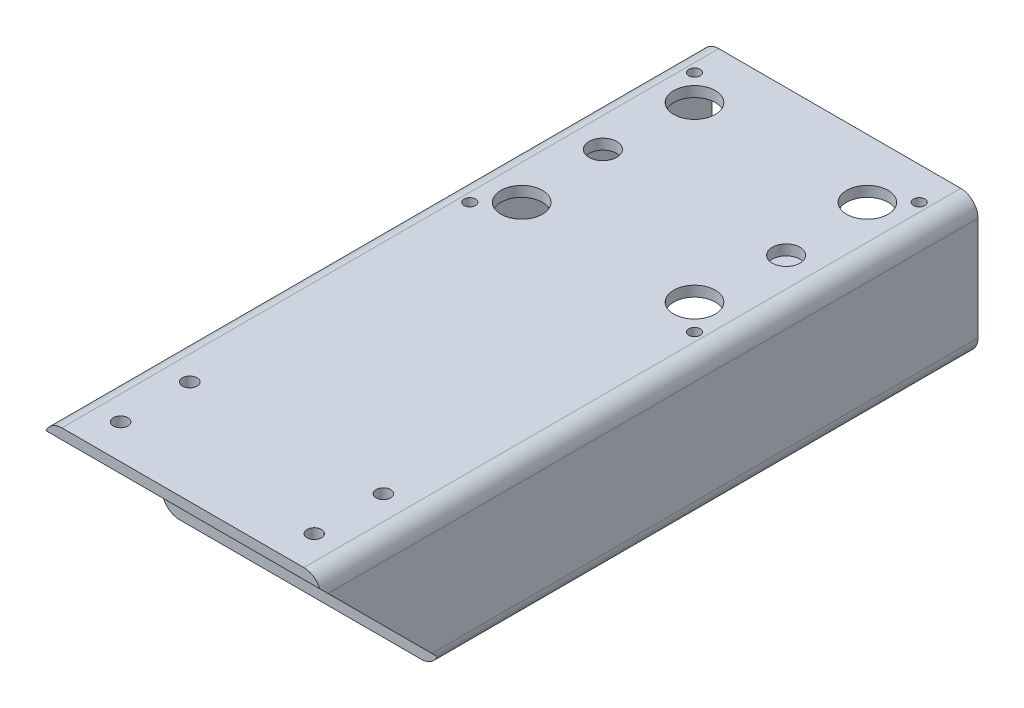
from build123d import *

# Parameters (mm, degrees)
EXTRUDE_1_DEPTH              = 190
SKETCH_6_R                   = 23.25
CUT_EXTRUDE_1_DEPTH          = 3
HOLE_WIZARD_6_5_6_5_1_D      = 6.5
HOLE_WIZARD_12_0_12_1_REACH  = 200.242
HOLE_WIZARD_12_0_12_1_BORE_R = 6
HOLE_WIZARD_M4_1_REACH       = 200.242
HOLE_WIZARD_M4_1_BORE_R      = 1.65
CUT_EXTRUDE_2_DEPTH          = 208.123151772
SKETCH_12_R                  = 5
EXTRUDE_2_DEPTH              = 3
HOLE_WIZARD_M5_1_D           = 4.2
HOLE_WIZARD_M3_1_D           = 2.5
HOLE_WIZARD_M3_1_DEPTH       = 3
CUT_EXTRUDE_3_REACH          = 200.242
SKETCH_17_R                  = 4


with BuildPart() as part:
    # 草图1 → 凸台-拉伸1 (new body)
    with BuildSketch(Plane.XY):
        with BuildLine():
            Line((-35, 20), (35, 20))
            ThreePointArc((35, 20), (38.535533906, 18.535533906), (40, 15))
            Line((40, 15), (40, -15))
            ThreePointArc((40, -15), (38.535533906, -18.535533906), (35, -20))
            Line((35, -20), (-35, -20))
            ThreePointArc((-35, -20), (-38.535533906, -18.535533906), (-40, -15))
            Line((-40, -15), (-40, 15))
            ThreePointArc((-40, 15), (-38.535533906, 18.535533906), (-35, 20))
        make_face()
        with BuildLine():
            Line((-37, 15), (-37, -15))
            ThreePointArc((-37, -15), (-36.414213562, -16.414213562), (-35, -17))
            Line((-35, -17), (35, -17))
            ThreePointArc((35, -17), (36.414213562, -16.414213562), (37, -15))
            Line((37, -15), (37, 15))
            ThreePointArc((37, 15), (36.414213562, 16.414213562), (35, 17))
            Line((35, 17), (-35, 17))
            ThreePointArc((-35, 17), (-36.414213562, 16.414213562), (-37, 15))
        make_face(mode=Mode.SUBTRACT)
    extrude(amount=EXTRUDE_1_DEPTH)

    # 草图6 → 切除-拉伸1 (cut)
    with BuildSketch(Plane.XZ.offset(20)):
        with Locations(Location((0, 42, 0), (0, 0, 270))):
            Circle(SKETCH_6_R)
    extrude(amount=-CUT_EXTRUDE_1_DEPTH, mode=Mode.SUBTRACT)

    # Ø6.5 (6.5) 直径孔1 (through all)
    with Locations(Plane(origin=(0, 20, 0), x_dir=(1, 0, 0), z_dir=(0, 1, 0))):
        with Locations((-25, -17), (25, -17), (25, -67), (-25, -67)):
            Hole(HOLE_WIZARD_6_5_6_5_1_D / 2)

    # Ø12.0 (12) 直径孔1 bore → Ø12.0 (12) 直径孔1 (cut, up to next)
    with BuildSketch(Plane(origin=(0, 20, 0), x_dir=(1, 0, 0), z_dir=(0, 1, 0)), mode=Mode.PRIVATE) as hole_wizard_12_0_12_1_sk1:
        with Locations((-25, -17)):
            Circle(HOLE_WIZARD_12_0_12_1_BORE_R)
    hole_wizard_12_0_12_1_tool1 = extrude(hole_wizard_12_0_12_1_sk1.sketch, amount=-HOLE_WIZARD_12_0_12_1_REACH, mode=Mode.PRIVATE) & part.part
    # Ø12.0 (12) 直径孔1 bore → Ø12.0 (12) 直径孔1 (cut, up to next)
    with BuildSketch(Plane(origin=(0, 20, 0), x_dir=(1, 0, 0), z_dir=(0, 1, 0)), mode=Mode.PRIVATE) as hole_wizard_12_0_12_1_sk2:
        with Locations((25, -17)):
            Circle(HOLE_WIZARD_12_0_12_1_BORE_R)
    hole_wizard_12_0_12_1_tool2 = extrude(hole_wizard_12_0_12_1_sk2.sketch, amount=-HOLE_WIZARD_12_0_12_1_REACH, mode=Mode.PRIVATE) & part.part
    # Ø12.0 (12) 直径孔1 bore → Ø12.0 (12) 直径孔1 (cut, up to next)
    with BuildSketch(Plane(origin=(0, 20, 0), x_dir=(1, 0, 0), z_dir=(0, 1, 0)), mode=Mode.PRIVATE) as hole_wizard_12_0_12_1_sk3:
        with Locations((25, -67)):
            Circle(HOLE_WIZARD_12_0_12_1_BORE_R)
    hole_wizard_12_0_12_1_tool3 = extrude(hole_wizard_12_0_12_1_sk3.sketch, amount=-HOLE_WIZARD_12_0_12_1_REACH, mode=Mode.PRIVATE) & part.part
    # Ø12.0 (12) 直径孔1 bore → Ø12.0 (12) 直径孔1 (cut, up to next)
    with BuildSketch(Plane(origin=(0, 20, 0), x_dir=(1, 0, 0), z_dir=(0, 1, 0)), mode=Mode.PRIVATE) as hole_wizard_12_0_12_1_sk4:
        with Locations((-25, -67)):
            Circle(HOLE_WIZARD_12_0_12_1_BORE_R)
    hole_wizard_12_0_12_1_tool4 = extrude(hole_wizard_12_0_12_1_sk4.sketch, amount=-HOLE_WIZARD_12_0_12_1_REACH, mode=Mode.PRIVATE) & part.part
    add(hole_wizard_12_0_12_1_tool1.solids().sort_by_distance((-25, 20, 17))[0], mode=Mode.SUBTRACT)
    add(hole_wizard_12_0_12_1_tool2.solids().sort_by_distance((25, 20, 17))[0], mode=Mode.SUBTRACT)
    add(hole_wizard_12_0_12_1_tool3.solids().sort_by_distance((25, 20, 67))[0], mode=Mode.SUBTRACT)
    add(hole_wizard_12_0_12_1_tool4.solids().sort_by_distance((-25, 20, 67))[0], mode=Mode.SUBTRACT)

    # M4 螺纹孔1 bore → M4 螺纹孔1 (cut, up to next)
    with BuildSketch(Plane(origin=(0, 20, 0), x_dir=(1, 0, 0), z_dir=(0, 1, 0)), mode=Mode.PRIVATE) as hole_wizard_m4_1_sk1:
        with Locations((-32.5, -9.5)):
            Circle(HOLE_WIZARD_M4_1_BORE_R)
    hole_wizard_m4_1_tool1 = extrude(hole_wizard_m4_1_sk1.sketch, amount=-HOLE_WIZARD_M4_1_REACH, mode=Mode.PRIVATE) & part.part
    # M4 螺纹孔1 bore → M4 螺纹孔1 (cut, up to next)
    with BuildSketch(Plane(origin=(0, 20, 0), x_dir=(1, 0, 0), z_dir=(0, 1, 0)), mode=Mode.PRIVATE) as hole_wizard_m4_1_sk2:
        with Locations((32.5, -9.5)):
            Circle(HOLE_WIZARD_M4_1_BORE_R)
    hole_wizard_m4_1_tool2 = extrude(hole_wizard_m4_1_sk2.sketch, amount=-HOLE_WIZARD_M4_1_REACH, mode=Mode.PRIVATE) & part.part
    # M4 螺纹孔1 bore → M4 螺纹孔1 (cut, up to next)
    with BuildSketch(Plane(origin=(0, 20, 0), x_dir=(1, 0, 0), z_dir=(0, 1, 0)), mode=Mode.PRIVATE) as hole_wizard_m4_1_sk3:
        with Locations((32.5, -74.5)):
            Circle(HOLE_WIZARD_M4_1_BORE_R)
    hole_wizard_m4_1_tool3 = extrude(hole_wizard_m4_1_sk3.sketch, amount=-HOLE_WIZARD_M4_1_REACH, mode=Mode.PRIVATE) & part.part
    # M4 螺纹孔1 bore → M4 螺纹孔1 (cut, up to next)
    with BuildSketch(Plane(origin=(0, 20, 0), x_dir=(1, 0, 0), z_dir=(0, 1, 0)), mode=Mode.PRIVATE) as hole_wizard_m4_1_sk4:
        with Locations((-32.5, -74.5)):
            Circle(HOLE_WIZARD_M4_1_BORE_R)
    hole_wizard_m4_1_tool4 = extrude(hole_wizard_m4_1_sk4.sketch, amount=-HOLE_WIZARD_M4_1_REACH, mode=Mode.PRIVATE) & part.part
    add(hole_wizard_m4_1_tool1.solids().sort_by_distance((-32.5, 20, 9.5))[0], mode=Mode.SUBTRACT)
    add(hole_wizard_m4_1_tool2.solids().sort_by_distance((32.5, 20, 9.5))[0], mode=Mode.SUBTRACT)
    add(hole_wizard_m4_1_tool3.solids().sort_by_distance((32.5, 20, 74.5))[0], mode=Mode.SUBTRACT)
    add(hole_wizard_m4_1_tool4.solids().sort_by_distance((-32.5, 20, 74.5))[0], mode=Mode.SUBTRACT)

    # 草图9 → 切除-拉伸2 (cut, through all)
    with BuildSketch(Plane(origin=(40, 0, 0), x_dir=(0, 0, -1), z_dir=(1, 0, 0))):
        Polygon((-190, 17), (-190, -20), (-156, -20), (-156, -17), align=None)
    extrude(amount=-CUT_EXTRUDE_2_DEPTH, mode=Mode.SUBTRACT)

    # 草图12 → 凸台-拉伸2 (add)
    with BuildSketch(Plane.XZ.offset(-17)):
        with Locations((-28, 160)):
            Circle(SKETCH_12_R)
        with Locations((-28, 180)):
            Circle(SKETCH_12_R)
        with Locations((28, 160)):
            Circle(SKETCH_12_R)
        with Locations((28, 180)):
            Circle(SKETCH_12_R)
    extrude(amount=EXTRUDE_2_DEPTH)

    # M5 螺纹孔1 (through all)
    with Locations(Plane(origin=(0, 20, 0), x_dir=(1, 0, 0), z_dir=(0, 1, 0))):
        with Locations((-28, -160), (-28, -180), (28, -160), (28, -180)):
            Hole(HOLE_WIZARD_M5_1_D / 2)

    # M3 螺纹孔1
    with Locations(Plane(origin=(0, -20, 0), x_dir=(-1, 0, 0), z_dir=(0, -1, 0))):
        with Locations((26.5, -42), (-26.5, -42)):
            Hole(HOLE_WIZARD_M3_1_D / 2, depth=HOLE_WIZARD_M3_1_DEPTH)

    # 草图17 → 切除-拉伸3 (cut, up to next)
    with BuildSketch(Plane(origin=(0, 20, 0), x_dir=(1, 0, 0), z_dir=(0, 1, 0)), mode=Mode.PRIVATE) as cut_extrude_3_sk1:
        with Locations(Location((-26.5, -42, 0), (0, 0, 270))):
            Circle(SKETCH_17_R)
    cut_extrude_3_tool1 = extrude(cut_extrude_3_sk1.sketch, amount=-CUT_EXTRUDE_3_REACH, mode=Mode.PRIVATE) & part.part
    # 草图17 → 切除-拉伸3 (cut, up to next)
    with BuildSketch(Plane(origin=(0, 20, 0), x_dir=(1, 0, 0), z_dir=(0, 1, 0)), mode=Mode.PRIVATE) as cut_extrude_3_sk2:
        with Locations(Location((26.5, -42, 0), (0, 0, 270))):
            Circle(SKETCH_17_R)
    cut_extrude_3_tool2 = extrude(cut_extrude_3_sk2.sketch, amount=-CUT_EXTRUDE_3_REACH, mode=Mode.PRIVATE) & part.part
    add(cut_extrude_3_tool1.solids().sort_by_distance((-26.5, 20, 42))[0], mode=Mode.SUBTRACT)
    add(cut_extrude_3_tool2.solids().sort_by_distance((26.5, 20, 42))[0], mode=Mode.SUBTRACT)


solid = part.part
